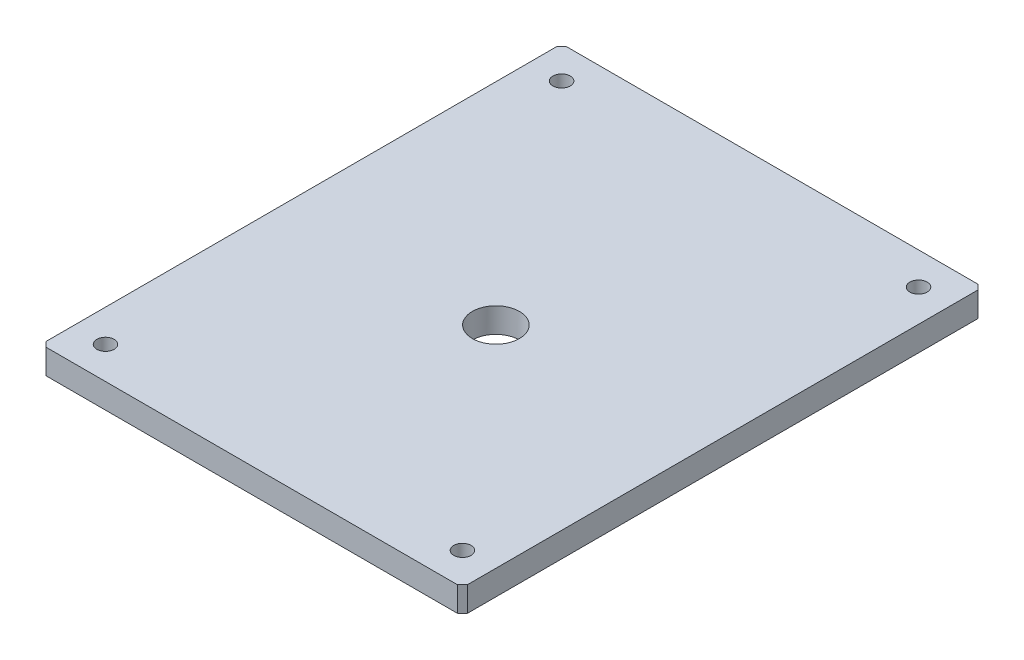
from build123d import *

# Parameters (mm, degrees)
SKETCH_1_W               = 170
SKETCH_1_H               = 210
EXTRUDE_1_DEPTH          = 10
CUT_EXTRUDE_1_REACH      = 137.462
SKETCH_2_R               = 9.5
CUT_EXTRUDE_2_REACH      = 137.462
SKETCH_3_R               = 3.5
MIRROR_2_COPY_1_REACH    = 137.462
MIRROR_2_COPY_1_SKETCH_R = 3.5
CHAMFER_1_SIZE           = 2


with BuildPart() as part:
    # 草图1 → 凸台-拉伸1 (new body)
    with BuildSketch(Plane(origin=(0, 0, 0), x_dir=(1, 0, 0), z_dir=(0, 1, 0))):
        Rectangle(SKETCH_1_W, SKETCH_1_H)
    extrude(amount=EXTRUDE_1_DEPTH)

    # 草图2 → 切除-拉伸1 (cut, up to next)
    with BuildSketch(Plane(origin=(0, 10, 0), x_dir=(1, 0, 0), z_dir=(0, 1, 0)), mode=Mode.PRIVATE) as cut_extrude_1_sk1:
        with Locations(Location((0, -6.5, 0), (0, 0, 270))):
            Circle(SKETCH_2_R)
    cut_extrude_1_tool1 = extrude(cut_extrude_1_sk1.sketch, amount=-CUT_EXTRUDE_1_REACH, mode=Mode.PRIVATE) & part.part
    add(cut_extrude_1_tool1.solids().sort_by_distance((0, 10, 6.5))[0], mode=Mode.SUBTRACT)

    # 草图3 → 切除-拉伸2 (cut, up to next)
    with BuildSketch(Plane.XZ, mode=Mode.PRIVATE) as cut_extrude_2_sk1:
        with Locations(Location((72, 92, 0), (0, 0, 270))):
            Circle(SKETCH_3_R)
    cut_extrude_2_tool1 = extrude(cut_extrude_2_sk1.sketch, amount=-CUT_EXTRUDE_2_REACH, mode=Mode.PRIVATE) & part.part
    cut_extrude_2 = cut_extrude_2_tool1.solids().sort_by_distance((72, 0, 92))[0]
    add(cut_extrude_2, mode=Mode.SUBTRACT)

    # 镜向1: 切除-拉伸2 across plane
    add(cut_extrude_2.mirror(Plane(origin=(0, 0, 0), x_dir=(0, 0, 1), z_dir=(1, 0, 0))), mode=Mode.SUBTRACT)

    # 镜向2: 切除-拉伸2 across plane
    add(cut_extrude_2.mirror(Plane.XY), mode=Mode.SUBTRACT)

    # 镜向2 copy 1 sketch → 镜向2 copy 1 (cut, up to next)
    with BuildSketch(Plane(origin=(0, 0, 0), x_dir=(-1, 0, 0), z_dir=(0, -1, 0)), mode=Mode.PRIVATE) as mirror_2_copy_1_sk1:
        with Locations(Location((72, 92, 0), (0, 0, 270))):
            Circle(MIRROR_2_COPY_1_SKETCH_R)
    mirror_2_copy_1_tool1 = extrude(mirror_2_copy_1_sk1.sketch, amount=-MIRROR_2_COPY_1_REACH, mode=Mode.PRIVATE) & part.part
    add(mirror_2_copy_1_tool1.solids().sort_by_distance((-72, 0, -92))[0], mode=Mode.SUBTRACT)

    # 倒角1
    chamfer_1_edges = [part.edges().sort_by_distance(p)[0] for p in [
        (85, 5, 105),
        (-85, 5, 105),
        (-85, 5, -105),
        (85, 5, -105),
    ]]
    chamfer(chamfer_1_edges, length=CHAMFER_1_SIZE)


solid = part.part
